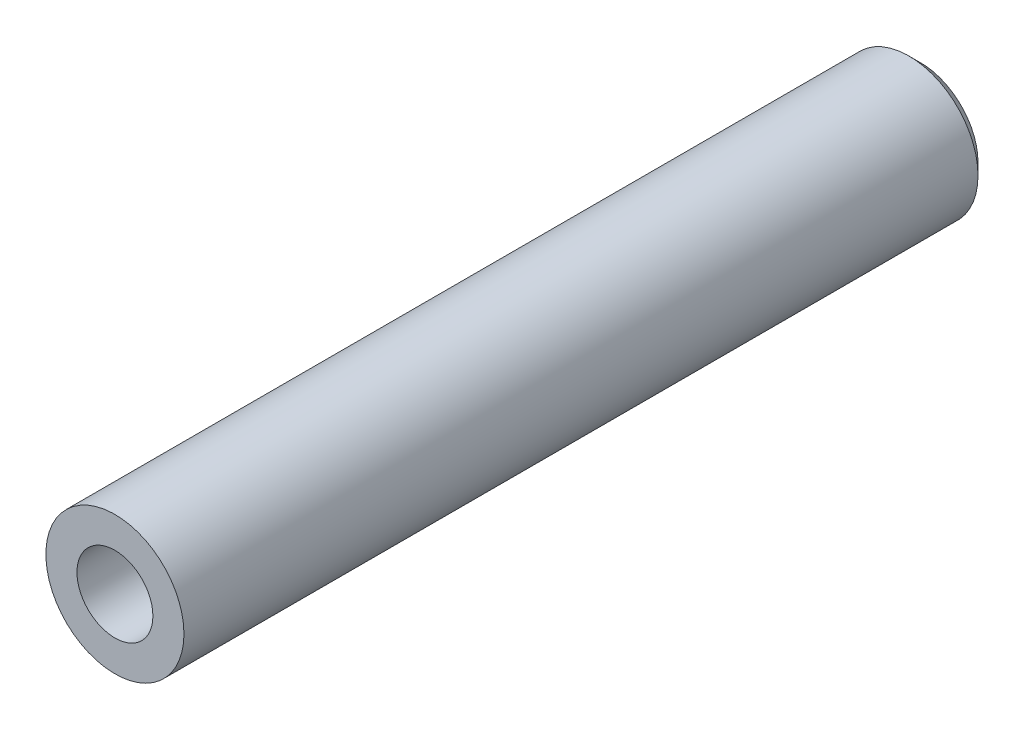
from build123d import *

# Parameters (mm, degrees)
SKETCH1_R             = 3
BOSS_EXTRUDE1_DEPTH   = 17.5
M4_TAPPED_HOLE1_D     = 3.3
M4_TAPPED_HOLE1_DEPTH = 10.1
M4_TAPPED_HOLE1_TIP   = 0.991420021
CHAMFER1_SIZE         = 0.5


with BuildPart() as part:
    # Sketch1 → Boss-Extrude1 (new, symmetric)
    with BuildSketch(Plane.XY):
        Circle(SKETCH1_R)
    extrude(amount=BOSS_EXTRUDE1_DEPTH, both=True)

    # M4 Tapped Hole1
    with Locations(Plane.XY.offset(17.5)):
        with Locations((0, 0)):
            Hole(M4_TAPPED_HOLE1_D / 2, depth=M4_TAPPED_HOLE1_DEPTH)
            with Locations((0, 0, -(M4_TAPPED_HOLE1_DEPTH + M4_TAPPED_HOLE1_TIP / 2))):  # 118° drill point
                Cone(0, M4_TAPPED_HOLE1_D / 2, M4_TAPPED_HOLE1_TIP, mode=Mode.SUBTRACT)

    # Chamfer1
    chamfer1_edges = [part.edges().sort_by_distance(p)[0] for p in [
        (-3, 0, -17.5),
    ]]
    chamfer(chamfer1_edges, length=CHAMFER1_SIZE)


solid = part.part
